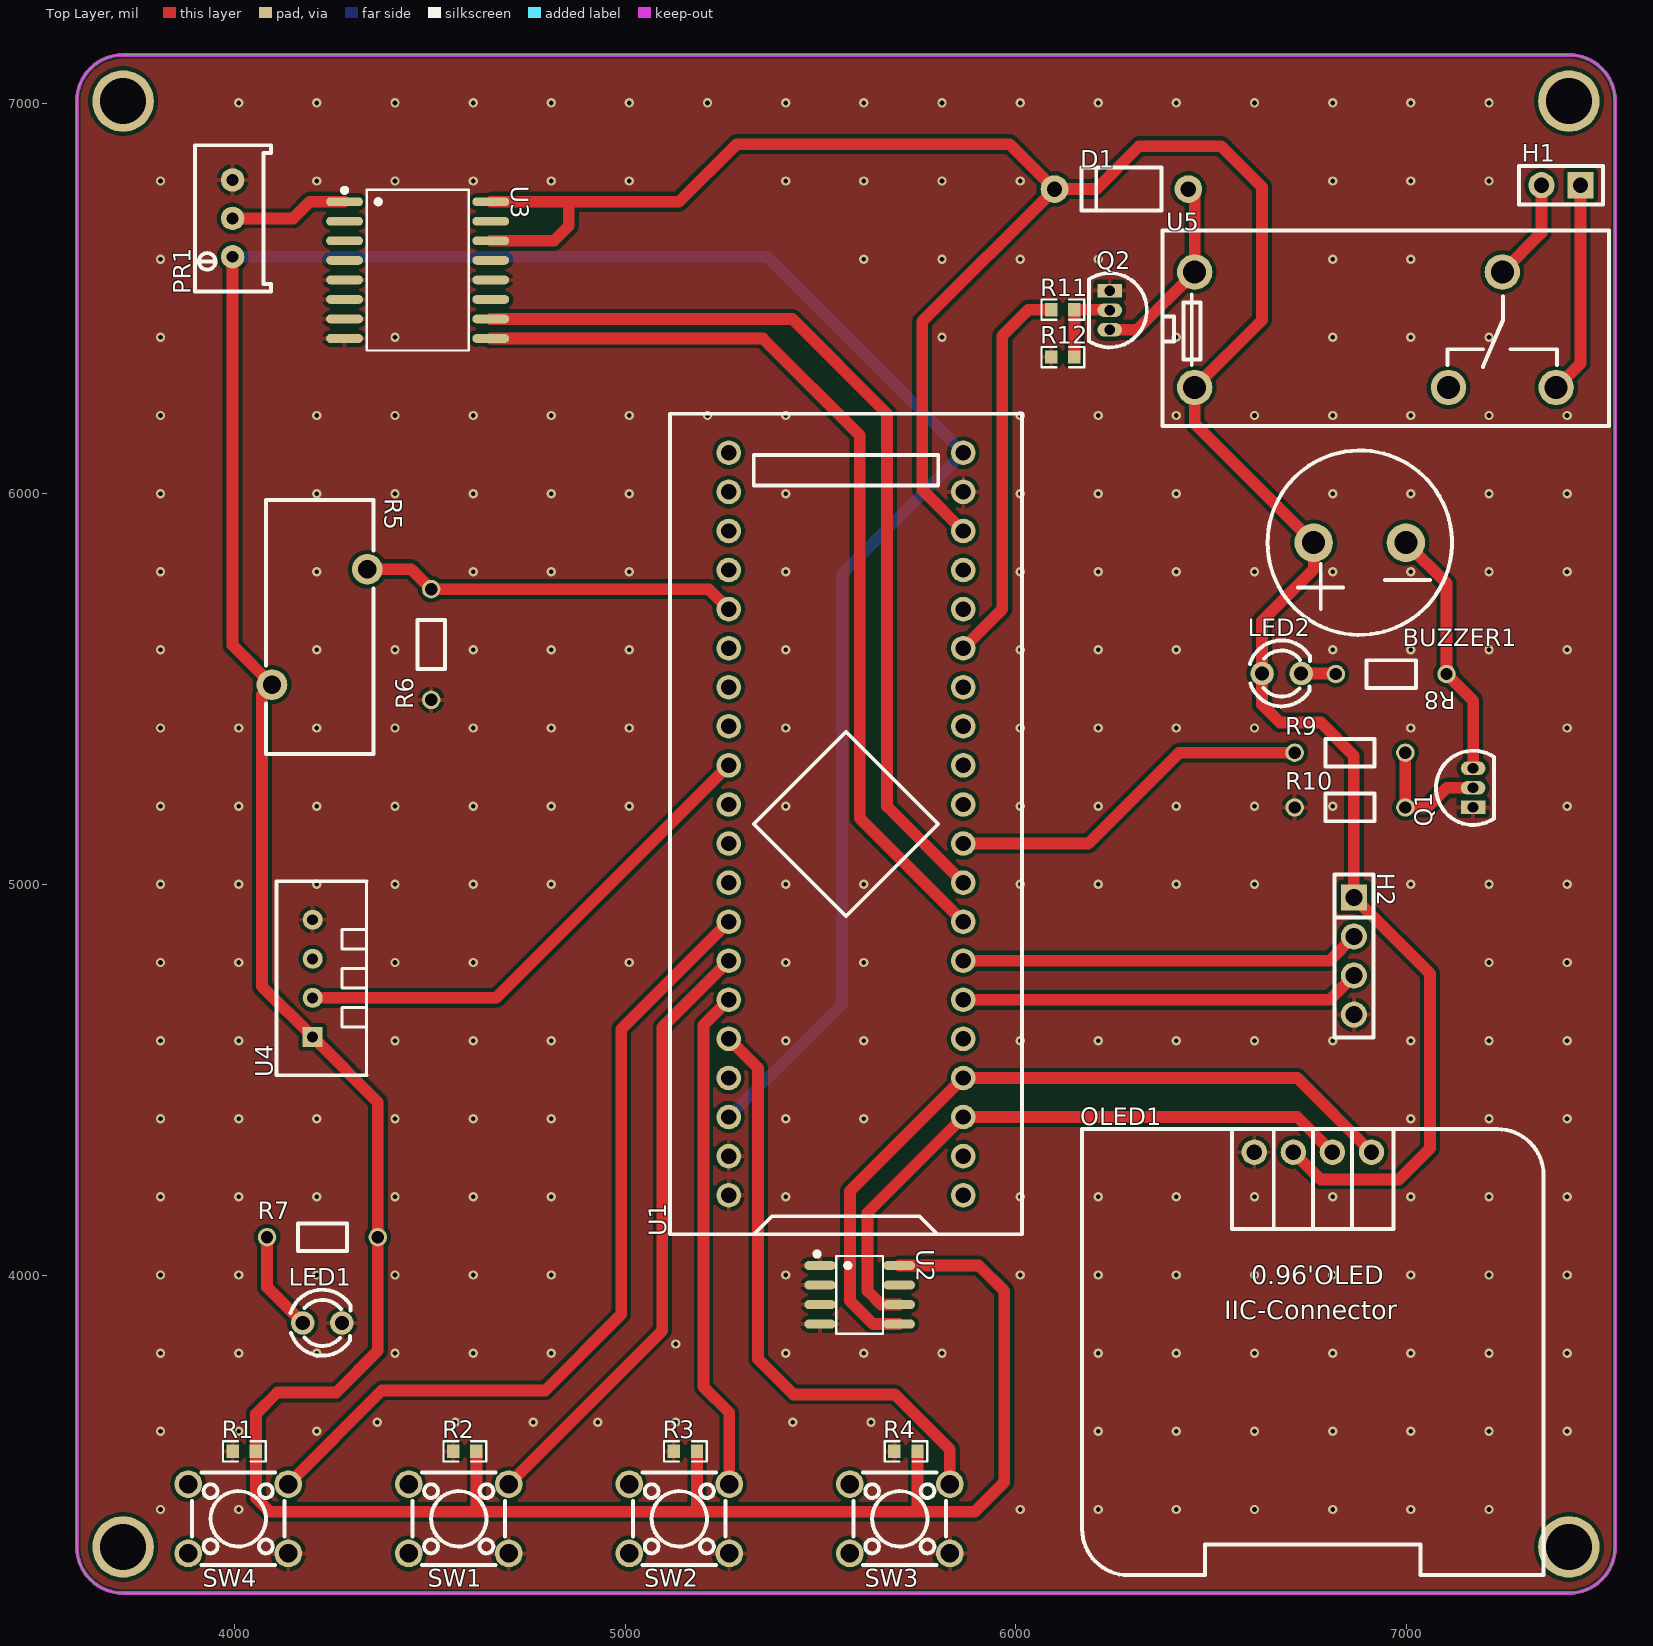
[diagram p0: Top Layer view]
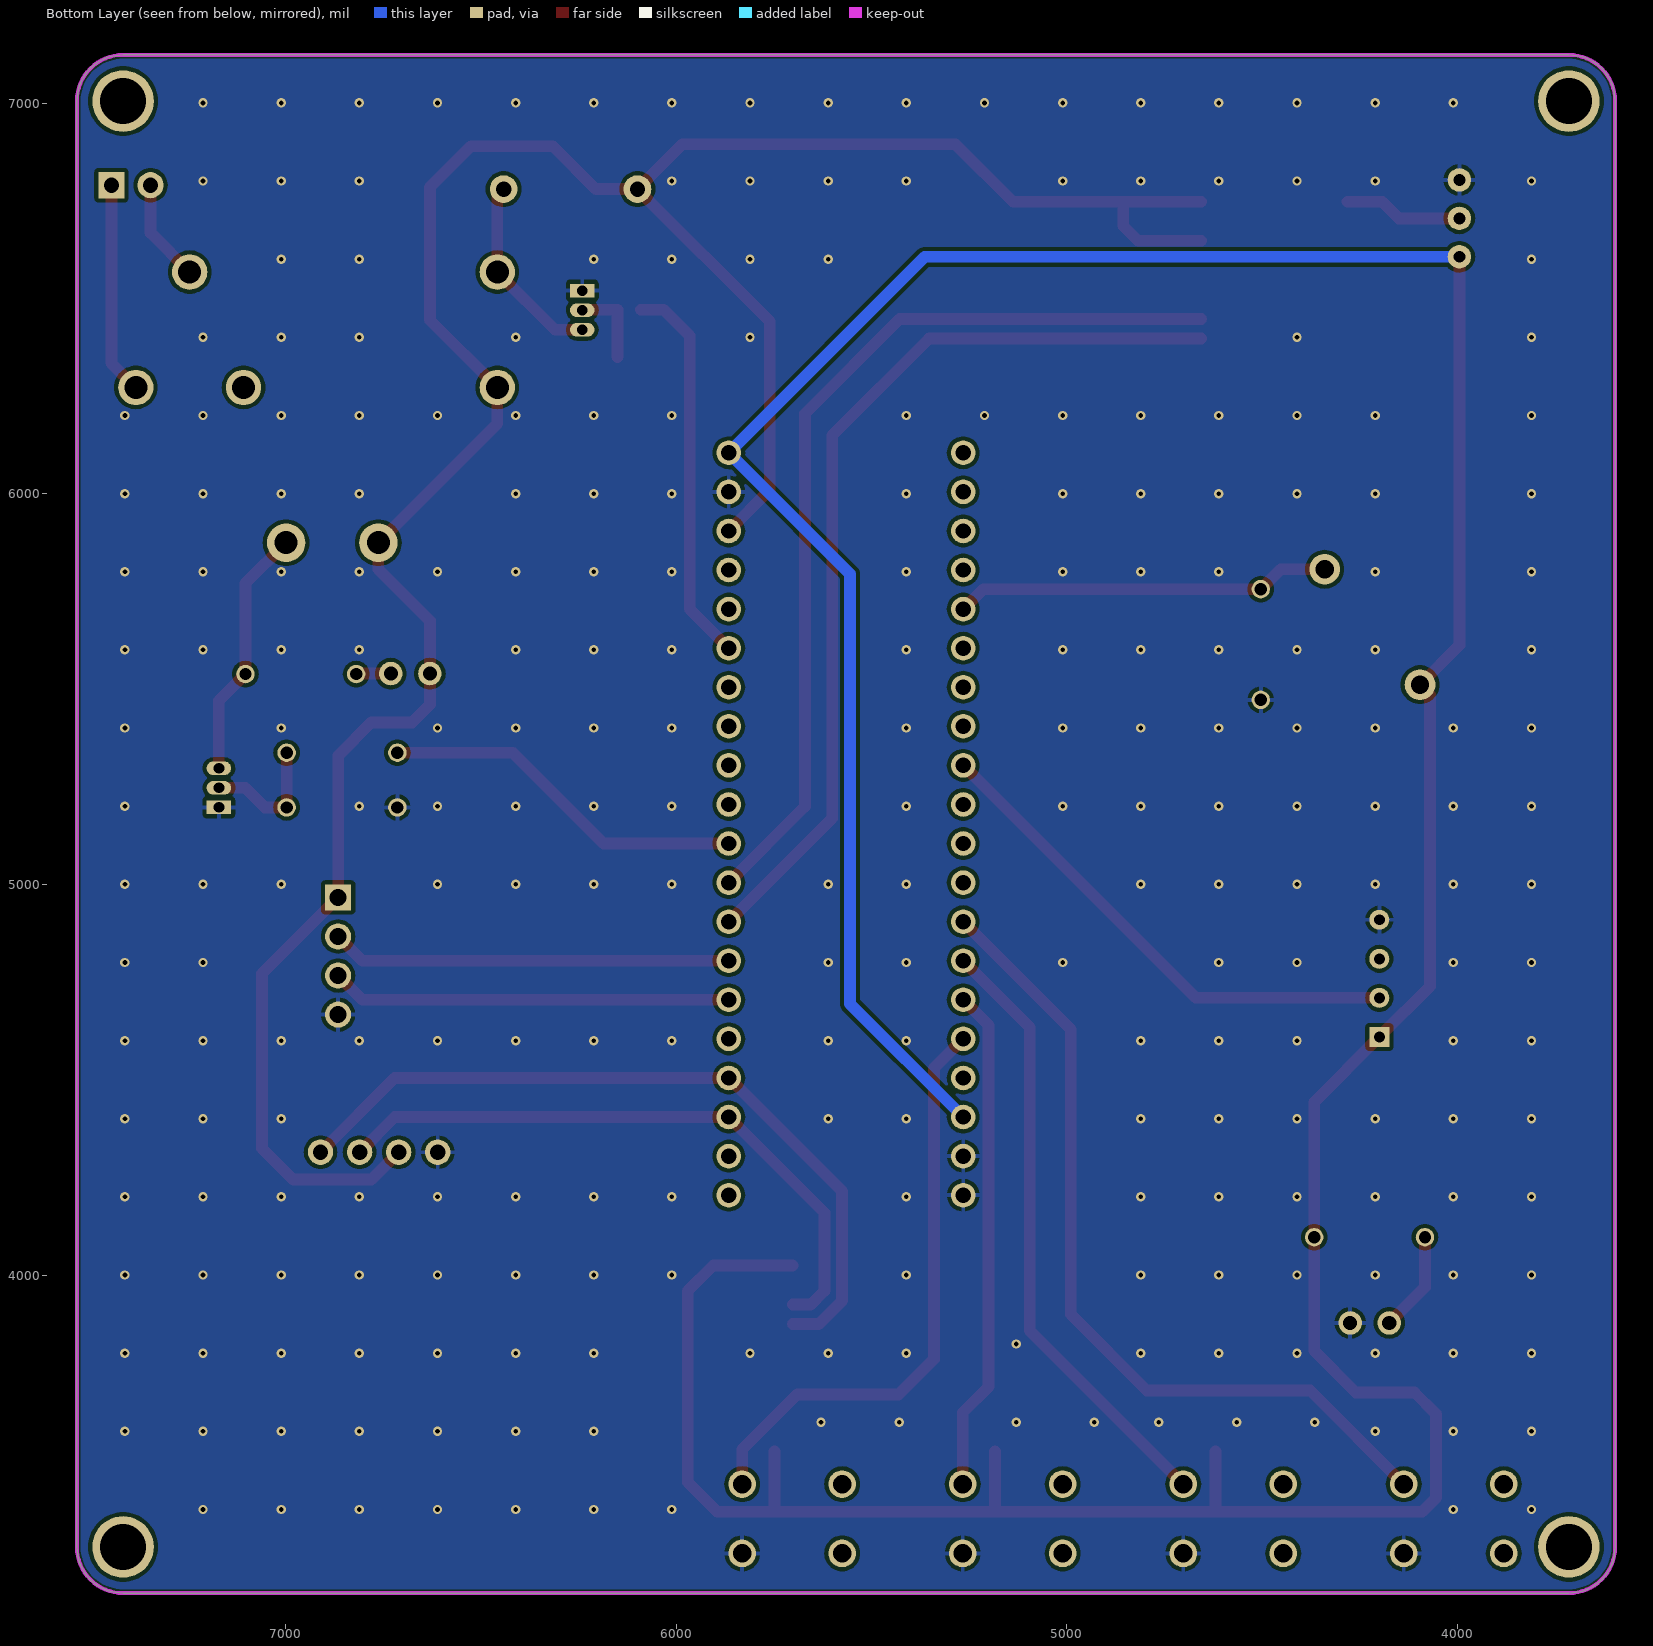
[diagram p1: Bottom Layer view, seen from below]
# Altium PCB MISC75094.pcbdoc
Units mil, origin at the board's own origin, x right, y up, seen from the top; angles counter-clockwise.
Board outline 3937.01 x 3937.01 mil, 2 copper layers (Top Layer, Bottom Layer), stack 62.206 mil thick; 31 components, 46 nets, 144 pads, 253 vias.

## Layer stack, top to bottom
Top Solder Mask Layer: solder mask 0.394, Dk 3.3
Top Layer: signal copper 1.379
Dielectric1: surface 59.449, FR4, Dk 4.5
Bottom Layer: signal copper 1.378
Bottom Solder Mask Layer: solder mask 0.394, Dk 3.3

## Board outline
3714.61,7123.5 ccw(c3714.61,7005.39) 3596.5,7005.39 3596.5,3304.61 ccw(c3714.61,3304.61) 3714.61,3186.5 7415.39,3186.5 ccw(c7415.39,3304.61) 7533.5,3304.61 7533.5,7005.39 ccw(c7415.39,7005.39) 7415.39,7123.5 3714.61,7123.5

## Design rules (kind name [scope] priority, off if disabled: settings)
BoardOutlineClearance copperThickness2oz_1 [All] p2 off: genericclearance=7.99 ignorepadtopadclearanceinfootprint=FALSE except(0: Arc-SplitContinuation Track-SplitContinuation SMDPad-SplitContinuation THPad-SplitContinuation Via-SplitContinuation Fill-SplitContinuation Region-SplitContinuation Poly-SplitContinuation Text-SplitContinuation Hole-SplitContinuation; 5.98: Arc-CutoutEdge Track-CutoutEdge SMDPad-CutoutEdge THPad-CutoutEdge Via-CutoutEdge Text-CutoutEdge; 6.9: Hole-OutlineEdge Hole-CutoutEdge; 10: Poly-OutlineEdge Poly-CutoutEdge; 11.81: Arc-OutlineEdge Track-OutlineEdge SMDPad-OutlineEdge THPad-OutlineEdge Via-OutlineEdge Fill-OutlineEdge Region-OutlineEdge Text-OutlineEdge Fill-CutoutEdge Region-CutoutEdge)
BoardOutlineClearance Plane_innerPlane_1 [All] p4 off: genericclearance=4.02 ignorepadtopadclearanceinfootprint=FALSE except(0: Arc-SplitContinuation Track-SplitContinuation SMDPad-SplitContinuation THPad-SplitContinuation Via-SplitContinuation Fill-SplitContinuation Region-SplitContinuation Poly-SplitContinuation Text-SplitContinuation Hole-SplitContinuation; 5.98: Arc-CutoutEdge Track-CutoutEdge SMDPad-CutoutEdge THPad-CutoutEdge Via-CutoutEdge Text-CutoutEdge; 6.9: Hole-OutlineEdge Hole-CutoutEdge; 10: Poly-OutlineEdge Poly-CutoutEdge; 11.81: Arc-OutlineEdge Track-OutlineEdge SMDPad-OutlineEdge THPad-OutlineEdge Via-OutlineEdge Fill-OutlineEdge Region-OutlineEdge Text-OutlineEdge Fill-CutoutEdge Region-CutoutEdge)
BoardOutlineClearance Copper_copperRegion_1 [All] p6 off: genericclearance=4.02 ignorepadtopadclearanceinfootprint=FALSE except(0: Arc-SplitContinuation Track-SplitContinuation SMDPad-SplitContinuation THPad-SplitContinuation Via-SplitContinuation Fill-SplitContinuation Region-SplitContinuation Poly-SplitContinuation Text-SplitContinuation Hole-SplitContinuation; 5.98: Arc-CutoutEdge Track-CutoutEdge SMDPad-CutoutEdge THPad-CutoutEdge Via-CutoutEdge Text-CutoutEdge; 6.9: Hole-OutlineEdge Hole-CutoutEdge; 10: Poly-OutlineEdge Poly-CutoutEdge; 11.81: Arc-OutlineEdge Track-OutlineEdge SMDPad-OutlineEdge THPad-OutlineEdge Via-OutlineEdge Fill-OutlineEdge Region-OutlineEdge Text-OutlineEdge Fill-CutoutEdge Region-CutoutEdge)
BoardOutlineClearance copperThickness1oz_1 [All] p8: genericclearance=4.02 ignorepadtopadclearanceinfootprint=FALSE except(0: Arc-SplitContinuation Track-SplitContinuation SMDPad-SplitContinuation THPad-SplitContinuation Via-SplitContinuation Fill-SplitContinuation Region-SplitContinuation Poly-SplitContinuation Text-SplitContinuation Hole-SplitContinuation; 5.98: Arc-CutoutEdge Track-CutoutEdge SMDPad-CutoutEdge THPad-CutoutEdge Via-CutoutEdge Text-CutoutEdge; 6.9: Hole-OutlineEdge Hole-CutoutEdge; 10: Poly-OutlineEdge Poly-CutoutEdge; 11.81: Arc-OutlineEdge Track-OutlineEdge SMDPad-OutlineEdge THPad-OutlineEdge Via-OutlineEdge Fill-OutlineEdge Region-OutlineEdge Text-OutlineEdge Fill-CutoutEdge Region-CutoutEdge)
Clearance copperThickness2oz [All] p1 off: gap=7.99 ignorepadtopadclearanceinfootprint=FALSE except(5.98: SMDPad-Track SMDPad-SMDPad THPad-Track SMDPad-THPad THPad-THPad Track-Via SMDPad-Via THPad-Via Via-Via Fill-SMDPad Region-SMDPad Fill-THPad Region-THPad Fill-Via Region-Via Fill-Fill Fill-Region Region-Region Arc-Track Arc-SMDPad Arc-THPad Arc-Via Fill-Arc Region-Arc Arc-Arc Text-Track SMDPad-Text Text-THPad Text-Via Fill-Text Region-Text Arc-Text Text-Text; 6.9: Hole-Track Hole-SMDPad Hole-THPad Hole-Via Fill-Hole Region-Hole Hole-Arc Hole-Text; 10: Poly-Track Poly-SMDPad Poly-THPad Poly-Via Poly-Fill Poly-Region Poly-Poly Poly-Arc Poly-Text Poly-Hole; 11.81: Fill-Track Region-Track)
Clearance Plane_innerPlane [All] p3 off: gap=4.02 ignorepadtopadclearanceinfootprint=FALSE except(5.98: SMDPad-Track SMDPad-SMDPad THPad-Track SMDPad-THPad THPad-THPad Track-Via SMDPad-Via THPad-Via Via-Via Fill-SMDPad Region-SMDPad Fill-THPad Region-THPad Fill-Via Region-Via Fill-Fill Fill-Region Region-Region Arc-Track Arc-SMDPad Arc-THPad Arc-Via Fill-Arc Region-Arc Arc-Arc Text-Track SMDPad-Text Text-THPad Text-Via Fill-Text Region-Text Arc-Text Text-Text; 6.9: Hole-Track Hole-SMDPad Hole-THPad Hole-Via Fill-Hole Region-Hole Hole-Arc Hole-Text; 10: Poly-Track Poly-SMDPad Poly-THPad Poly-Via Poly-Fill Poly-Region Poly-Poly Poly-Arc Poly-Text Poly-Hole; 11.81: Fill-Track Region-Track)
Clearance Copper_copperRegion [All] p5 off: gap=4.02 ignorepadtopadclearanceinfootprint=FALSE except(5.98: SMDPad-Track SMDPad-SMDPad THPad-Track SMDPad-THPad THPad-THPad Track-Via SMDPad-Via THPad-Via Via-Via Fill-SMDPad Region-SMDPad Fill-THPad Region-THPad Fill-Via Region-Via Fill-Fill Fill-Region Region-Region Arc-Track Arc-SMDPad Arc-THPad Arc-Via Fill-Arc Region-Arc Arc-Arc Text-Track SMDPad-Text Text-THPad Text-Via Fill-Text Region-Text Arc-Text Text-Text; 6.9: Hole-Track Hole-SMDPad Hole-THPad Hole-Via Fill-Hole Region-Hole Hole-Arc Hole-Text; 10: Poly-Track Poly-SMDPad Poly-THPad Poly-Via Poly-Fill Poly-Region Poly-Poly Poly-Arc Poly-Text Poly-Hole; 11.81: Fill-Track Region-Track)
Clearance copperThickness1oz [All] p7: gap=4.02 ignorepadtopadclearanceinfootprint=FALSE except(5.98: SMDPad-Track SMDPad-SMDPad THPad-Track SMDPad-THPad THPad-THPad Track-Via SMDPad-Via THPad-Via Via-Via Fill-SMDPad Region-SMDPad Fill-THPad Region-THPad Fill-Via Region-Via Fill-Fill Fill-Region Region-Region Arc-Track Arc-SMDPad Arc-THPad Arc-Via Fill-Arc Region-Arc Arc-Arc Text-Track SMDPad-Text Text-THPad Text-Via Fill-Text Region-Text Arc-Text Text-Text; 6.9: Hole-Track Hole-SMDPad Hole-THPad Hole-Via Fill-Hole Region-Hole Hole-Arc Hole-Text; 10: Poly-Track Poly-SMDPad Poly-THPad Poly-Via Poly-Fill Poly-Region Poly-Poly Poly-Arc Poly-Text Poly-Hole; 11.81: Fill-Track Region-Track)
DiffPairsRouting differentialPair [All] p1: maxlimit=6 minlimit=6 mostfreqgap=6 toplayer_minwidth=5 toplayer_prefwidth=10 toplayer_maxwidth=100 toplayer_mingap=6 toplayer_prefgap=6 toplayer_maxgap=6 bottomlayer_minwidth=5 bottomlayer_prefwidth=10 bottomlayer_maxwidth=100 bottomlayer_mingap=6 bottomlayer_prefgap=6 bottomlayer_maxgap=6 maxuncoupledlength=10
HoleToHoleClearance otherClearance [All] p1: gap=11.81 allowstackedmicrovias=TRUE
Length netLength [All] p1: minlimit=0 maxlimit=0
PasteMaskExpansion pasteMaskExpansion [All] p1: expansion=0
PlaneConnect innerPlane [All] p1: planeconnectstyle=Relief reliefexpansion=20 reliefentries=4 reliefconductorwidth=10 reliefairgap=10
PolygonConnect copperRegion [All] p1: connectstyle=Relief reliefconductorwidth=10 reliefentries=4 polygonreliefangle="90 Angle" airgapwidth=10 via.connectstyle=Relief via.reliefconductorwidth=10 via.reliefentries=4 via.polygonreliefangle="90 Angle" via.airgapwidth=10
RoutingVias viaSize [All] p1: holewidth=12.01 width=24.02 viastyle="Through Hole" minholewidth=11.81 minwidth=19.68 maxholewidth=248.03 maxwidth=393.7
SolderMaskExpansion solderMaskExpansion [IsVia] p1: expansion=-1000 istentingtop=TRUE
SolderMaskExpansion solderMaskExpansion [All] p2: expansion=2 istentingtop=FALSE
Width copperThickness2oz_2 [All] p1 off: maxlimit=100 minlimit=8 preferedwidth=10
Width copperThickness1oz_2 [All] p2: maxlimit=100 minlimit=5 preferedwidth=10

## Components (designator, comment, footprint, x,y, rotation, side; value= is the part's Value field where it differs from the comment)
BUZZER1 "buzzer" BUZ-TH_BD12.0-P6.00-D0.9-RD 6880,5875 r180 top
D1 "" DO_1N4007 6270,6780 r0 top
H1 "" HDR-TH_2P-P2.54-V-F 7395,6790 r180 top
H2 "" HDR-TH_4P-P2.54-V-F 6864.9,4817.04 r270 top
LED1 "" LED_TH-3mm 4224.65,3877.95 r0 top
LED2 "" LED_TH-3mm 6680,5540 r0 top
OLED1 "" 0.96OLED_4P 6760,4315 r0 top
PR1 "10kΩ" R_3296 3990,6705 r90 top
Q1 "" S8050_TO_92 7170.1,5247.66 r90 top
Q2 "" S8050_TO_92 6240,6470 r270 top
R1 "10K" R0603 4025.08,3549.45 r0 top
R2 "10K" R0603 4589.49,3549.45 r0 top
R3 "10K" R0603 5153.9,3549.45 r0 top
R4 "10K" R0603 5718.32,3549.45 r0 top
R5 "3Ω,7A,0.075Ω" RES-TH_L16.5-W7.0-P7.50-D0.8-S6.2 4217.88,5659.29 r270 top
R6 "10kΩ" Res_1/8W 4505.81,5614.38 r90 top
R7 "500Ω" Res_1/8W 4225,4095 r0 top
R8 "10Ω" Res_1/8W 6960.41,5541.25 r180 top
R9 "1kΩ" Res_1/8W 6855,5335 r0 top
R10 "10kΩ" Res_1/8W 6855,5195 r0 top
R11 "1K" R0603 6119.85,6471.25 r0 top
R12 "10K" R0603 6120,6350 r0 top
SW1 "" SW-TH_4P-L6.0-W6.0-P4.50-LS6.5 4573.89,3376.74 r180 top
SW2 "" SW-TH_4P-L6.0-W6.0-P4.50-LS6.5 5138.3,3376.74 r180 top
SW3 "" SW-TH_4P-L6.0-W6.0-P4.50-LS6.5 5702.72,3376.74 r180 top
SW4 "" SW-TH_4P-L6.0-W6.0-P4.50-LS6.5 4009.48,3376.74 r180 top
U1 "STM32F103C8T6-Card" CONN-TH_L53.3-W22.9_STM32F103C8T6-CARD 5565,5155 r90 top
U2 "24C02CT-I/SN" SOIC-8_L4.9-W3.9-P1.27-LS6.0-BL 5600,3950 r270 top
U3 "PCF8591T" SOIC-16_L10.3-W7.5-P1.27-LS10.3-BL 4468.71,6572.61 r270 top
U4 "DHT11" SENSOR-TH_DHT11 4200,4760 r90 top
U5 "SSKD6132" RELAY-TH_G2R-1 6920,6420 r0 top

## Footprints (in the part's own frame and the unit in brackets; to place one, negate y for a bottom-side part, rotate by r counter-clockwise, add the part's x,y. Pads: shape width x height; smd on the part's side, far side on the other; paste and mask are expansions set on the pad)
0.96OLED_4P [mm]
  round 1.65 hole 1 copper offset 0,0: 1(-3.81,-0.001) 2(-1.27,0.002) 3(1.27,0.002) 4(3.81,0.002)
  silkscreen extent -15,-27.5 15,1.5
BUZ-TH_BD12.0-P6.00-D0.9-RD [mm]
  round 2.5 hole 1.5 paste+0 mask+0.05: 1(-3,0) 2(3,0)
  silkscreen extent -5.99,-5.99 5.99,5.99
CONN-TH_L53.3-W22.9_STM32F103C8T6-CARD [mm]
  round 1.6 hole 1: 1(-24.13,-7.62) 2(-21.59,-7.62) 3(-19.05,-7.62) 4(-16.51,-7.62) 5(-13.97,-7.62) 6(-11.43,-7.62) 7(-8.89,-7.62) 8(-6.35,-7.62) 9(-3.81,-7.62) 10(-1.27,-7.62) 11(1.27,-7.62) 12(3.81,-7.62) 13(6.35,-7.62) 14(8.89,-7.62) 15(11.43,-7.62) 16(13.97,-7.62) 17(16.51,-7.62) 18(19.05,-7.62) 19(21.59,-7.62) 20(24.13,-7.62) 21(24.13,7.62) 22(21.59,7.62) 23(19.05,7.62) 24(16.51,7.62) 25(13.97,7.62) 26(11.43,7.62) 27(8.89,7.62) 28(6.35,7.62) 29(3.81,7.62) 30(1.27,7.62) 31(-1.27,7.62) 32(-3.81,7.62) 33(-6.35,7.62) 34(-8.89,7.62) 35(-11.43,7.62) 36(-13.97,7.62) 37(-16.51,7.62) 38(-19.05,7.62) 39(-21.59,7.62) 40(-24.13,7.62)
  silkscreen extent -26.67,-11.43 26.67,11.43
DO_1N4007 [mm]
  round 1.8 hole 1 paste+0 mask+0.051: 1(-4.35,0) 2(4.35,0)
  silkscreen extent -2.6,-1.4 2.6,1.4
HDR-TH_2P-P2.54-V-F [mm]
  rect 1.7x1.7 hole 1: 1(-1.27,0)
  round 1.7 hole 1: 2(1.27,0)
  silkscreen extent -2.74,-1.25 2.74,1.25
HDR-TH_4P-P2.54-V-F [mm]
  rect 1.7x1.7 hole 1.1: 1(-3.81,0)
  round 1.7 hole 1.1: 2(-1.27,0) 3(1.27,0) 4(3.81,0)
  silkscreen extent -5.29,-1.27 5.29,1.27
LED_TH-3mm [mil]
  round 60 hole 36 paste+0 mask+2: 1(-50,0) 2(50,0)
  silkscreen extent -81,-84 72,85
R0603 [mil]
  rect 31.75x34.02 smd paste-3937.01 mask+2: 1(-29.66,0) 2(29.66,0)
  silkscreen extent -55,-26 55,26
R_3296 [mil]
  round 60 hole 30 paste+0 mask+2: 1(-98.4,-5) 2(0,-5) 3(98.4,-5)
  silkscreen extent -187,-103 187,92
RELAY-TH_G2R-1 [mm]
  round 2.3 hole 1.5: 1(-11.75,-3.75) 2(4.75,-3.75) 3(11.75,-3.75) 4(8.25,3.75) 5(-11.75,3.75)
  silkscreen extent -13.83,-6.26 15.17,6.44
RES-TH_L16.5-W7.0-P7.50-D0.8-S6.2 [mm]
  round 2 hole 1.2: 1(-3.75,3.1) 2(3.75,-3.1)
  silkscreen extent -8.25,-3.5 8.25,3.5
Res_1/8W [mil]
  round 47.2 hole 31.5 paste+0 mask+2: 1(-141.7,2.48) 2(141.7,2.48)
  silkscreen extent -63,-33 63,38
S8050_TO_92 [mil]
  rect 35.4x63 hole 27.6 paste+0 mask+2: 1(-50,0)
  oval 35.4x63 hole 27.6 paste+0 mask+2: 2(0,0) 3(50,0)
  silkscreen extent -95,-53 95,95
SENSOR-TH_DHT11 [mil]
  rect 51x51 hole 28: 1(-150,0)
  round 51 hole 28: 2(-50,0) 3(50,0) 4(150,0)
  silkscreen extent -248,-138 248,93
SOIC-8_L4.9-W3.9-P1.27-LS6.0-BL [mm]
  oval 0.588x2.045 smd: 1(-1.905,-2.57) 2(-0.635,-2.57) 3(0.635,-2.57) 4(1.905,-2.57) 5(1.905,2.57) 6(0.635,2.57) 7(-0.635,2.57) 8(-1.905,2.57)
  silkscreen extent -2.8,-2.92 2.53,1.52
SOIC-16_L10.3-W7.5-P1.27-LS10.3-BL [mil]
  oval 22.6x94.51 smd: 1(-175,-187.02) 2(-125,-187.02) 3(-75,-187.02) 4(-25,-187.02) 5(25,-187.02) 6(75,-187.02) 7(125,-187.02) 8(175,-187.02) 9(175,187.02) 10(125,187.02) 11(75,187.02) 12(25,187.02) 13(-25,187.02) 14(-75,187.02) 15(-125,187.02) 16(-175,187.02)
  silkscreen extent -210,-193 206,131
SW-TH_4P-L6.0-W6.0-P4.50-LS6.5 [mm]
  round 1.8 hole 1.2: 1(-3.25,2.25) 2(3.25,2.25) 3(-3.25,-2.25) 4(3.25,-2.25)
  silkscreen extent -3,-3 3,3

## Free pads (board coordinates)
  round 157.48 hole 118.11: 1(3714.61,7005.39) 1(3714.61,3304.61) 1(7415.39,7005.39) 1(7415.39,3304.61)

## Via types
v1: diameter 24.02, hole 12, Top Layer to Bottom Layer, 253 vias

## Nets (pads, with @x,y where several pads share a name; then routed paths per layer and width w, separated by ;. In a path a pad name is that pad's centre, name@x,y a point inside that pad or via, vN(x,y) a via of type N, cw(c..) or ccw(c..) an arc to the next point about the centre after c; other vN are vias at no path point)
$1N17153: LED1.1 R7.1 | length 257.4
  Top Layer w30: R7.1 4083.3,3969.3 LED1.1
$1N17160: PR1.2 U3.1 | length 314.3
  Top Layer w30: PR1.2@3985,6705 4150,6705 4192.61,6747.61 U3.1
$1N17168: BUZZER1.1 Q1.3 R8.1 | length 648.6
  Top Layer w30: BUZZER1.1 7102.11,5771 R8.1 7170.1,5470.79 Q1.3
$1N17169: Q1.2 R9.2 R10.2 | length 334.2
  Top Layer w30: R9.2 R10.2 7052.48,5197.48 7102.66,5247.66 Q1.2
$1N17173: LED2.2 R8.2 | length 89.2
  Top Layer w30: LED2.2 6817.49,5540 R8.2
$1N17174: D1.2 Q2.3 U5.5 | length 497.6
  Top Layer w30: Q2.3 6309.75,6420 U5.5 6457.4,6763.86 D1.2
$1N17176: Q2.2 R11.2 R12.2 | length 212.3
  Top Layer w30: R12.2 6149.66,6471.1 R11.2 6238.75,6471.25 Q2.2
$1N17179: H1.2 U5.4 | length 263.9
  Top Layer w30: U5.4 7345,6667.85 H1.2
$1N17180: H1.1 U5.3 | length 543.5
  Top Layer w30: U5.3 7445,6334.75 H1.1
+5V: BUZZER1.2 D1.1 H2.1 LED2.1 OLED1.2 U1.18 U3.14 U3.16 U5.1 | length 6872.4
  Top Layer w30: U3.14 4817.61,6647.61 4855.55,6685.55 4855.55,6747.61 ; U3.16 4855.55,6747.61 ; U1.18 5760,6010 5760,6441.26 D1.1 ; OLED1.2@6710,4315.05 6780.05,4245 6980,4245 7060,4325 7060,4771.94 H2.1 6864.9,5330.1 6780,5415 6675,5415 6630,5460 LED2.1 6630,5675 6761.89,5806.89 BUZZER1.2 6457.4,6179.49 U5.1 6630,6444.95 6630,6785 6525,6890 6315,6890 6205,6780 D1.1 ; 4855.55,6747.61 5137.61,6747.61 5285,6895 5983.74,6895 D1.1
BUZZER: R9.1 U1.10 | length 944.6
  Top Layer w30: U1.10 6185,5105 6417.48,5337.48 R9.1
DATA: U1.29 U4.2 | length 1311.5
  Top Layer w30: U4.2 4670,4710 U1.29
GND: H2.4 LED1.2 OLED1.1 PR1.3 Q1.1 Q2.1 R1.1 R2.1 R3.1 R4.1 R6.1 R10.1 R12.1 SW1.1 SW2.1 SW3.1 SW4.1 U1.19 U1.39 U1.40 U2.1 U2.2 U2.3 U2.4 U3.5 U3.6 U3.7 U3.8 U3.12 U4.4
  other v1: 3810.6,3400.6 4010.6,3400.6 6010.6,3400.6 6210.6,3400.6 6410.6,3400.6 6610.6,3400.6 6810.6,3400.6 7010.6,3400.6 7210.6,3400.6 3810.6,3600.6 4010.6,3600.6 4210.6,3600.6 6210.6,3600.6 6410.6,3600.6 6610.6,3600.6 6810.6,3600.6 7010.6,3600.6 7210.6,3600.6 7410.6,3600.6 4364.89,3624.1 4564.89,3624.1 4764.89,3624.1 4929.3,3624.1 5129.3,3624.1 5429.1,3624.1 5629.1,3624.1 3810.6,3800.6 4010.6,3800.6 4210.6,3800.6 4410.6,3800.6 4610.6,3800.6 4810.6,3800.6 5410.6,3800.6 5610.6,3800.6 5810.6,3800.6 6210.6,3800.6 6410.6,3800.6 6610.6,3800.6 6810.6,3800.6 7010.6,3800.6 7210.6,3800.6 7410.6,3800.6 5129.3,3824.1 3810.6,4000.6 4010.6,4000.6 4210.6,4000.6 4410.6,4000.6 4610.6,4000.6 4810.6,4000.6 5410.6,4000.6 6010.6,4000.6 6210.6,4000.6 6410.6,4000.6 6610.6,4000.6 6810.6,4000.6 7010.6,4000.6 7210.6,4000.6 7410.6,4000.6 3810.6,4200.6 4010.6,4200.6 4210.6,4200.6 4410.6,4200.6 4610.6,4200.6 4810.6,4200.6 5410.6,4200.6 6010.6,4200.6 6210.6,4200.6 6410.6,4200.6 6610.6,4200.6 6810.6,4200.6 7010.6,4200.6 7210.6,4200.6 7410.6,4200.6 3810.6,4400.6 4010.6,4400.6 4210.6,4400.6 4410.6,4400.6 4610.6,4400.6 4810.6,4400.6 5410.6,4400.6 5610.6,4400.6 7010.6,4400.6 7210.6,4400.6 7410.6,4400.6 3810.6,4600.6 4010.6,4600.6 4410.6,4600.6 4610.6,4600.6 4810.6,4600.6 5410.6,4600.6 5610.6,4600.6 6010.6,4600.6 6210.6,4600.6 6410.6,4600.6 6610.6,4600.6 6810.6,4600.6 7010.6,4600.6 7210.6,4600.6 7410.6,4600.6 3810.6,4800.6 4010.6,4800.6 4410.6,4800.6 4610.6,4800.6 5010.6,4800.6 5410.6,4800.6 5610.6,4800.6 7210.6,4800.6 7410.6,4800.6 3810.6,5000.6 4010.6,5000.6 4210.6,5000.6 4410.6,5000.6 4610.6,5000.6 4810.6,5000.6 5410.6,5000.6 5610.6,5000.6 6010.6,5000.6 6210.6,5000.6 6410.6,5000.6 6610.6,5000.6 7010.6,5000.6 7210.6,5000.6 7410.6,5000.6 3810.6,5200.6 4010.6,5200.6 4210.6,5200.6 4410.6,5200.6 4610.6,5200.6 4810.6,5200.6 5010.6,5200.6 5410.6,5200.6 6010.6,5200.6 6210.6,5200.6 6410.6,5200.6 6610.6,5200.6 6810.6,5200.6 7410.6,5200.6 3810.6,5400.6 4010.6,5400.6 4210.6,5400.6 4410.6,5400.6 4610.6,5400.6 4810.6,5400.6 5010.6,5400.6 5410.6,5400.6 6010.6,5400.6 6210.6,5400.6 6410.6,5400.6 6610.6,5400.6 7010.6,5400.6 7410.6,5400.6 3810.6,5600.6 4210.6,5600.6 4410.6,5600.6 4610.6,5600.6 4810.6,5600.6 5010.6,5600.6 5410.6,5600.6 6010.6,5600.6 6210.6,5600.6 6410.6,5600.6 6810.6,5600.6 7010.6,5600.6 7210.6,5600.6 7410.6,5600.6 3810.6,5800.6 4210.6,5800.6 4610.6,5800.6 4810.6,5800.6 5010.6,5800.6 5410.6,5800.6 6010.6,5800.6 6210.6,5800.6 6410.6,5800.6 6610.6,5800.6 6810.6,5800.6 7010.6,5800.6 7210.6,5800.6 7410.6,5800.6 3810.6,6000.6 4210.6,6000.6 4410.6,6000.6 4610.6,6000.6 4810.6,6000.6 5010.6,6000.6 5410.6,6000.6 6010.6,6000.6 6210.6,6000.6 6410.6,6000.6 6810.6,6000.6 7010.6,6000.6 7210.6,6000.6 7410.6,6000.6 3810.6,6200.6 4210.6,6200.6 4410.6,6200.6 4610.6,6200.6 4810.6,6200.6 5010.6,6200.6 5210.6,6200.6 5410.6,6200.6 6010.6,6200.6 6210.6,6200.6 6410.6,6200.6 6610.6,6200.6 6810.6,6200.6 7010.6,6200.6 7210.6,6200.6 7410.6,6200.6 3810.6,6400.6 4410.6,6400.6 5810.6,6400.6 6410.6,6400.6 6810.6,6400.6 7010.6,6400.6 7210.6,6400.6 3810.6,6600.6 5610.6,6600.6 5810.6,6600.6 6010.6,6600.6 6210.6,6600.6 6810.6,6600.6 7010.6,6600.6 3810.6,6800.6 4210.6,6800.6 4410.6,6800.6 4610.6,6800.6 4810.6,6800.6 5010.6,6800.6 5410.6,6800.6 5610.6,6800.6 5810.6,6800.6 6010.6,6800.6 6810.6,6800.6 7010.6,6800.6 7210.6,6800.6 4010.6,7000.6 4210.6,7000.6 4410.6,7000.6 4610.6,7000.6 4810.6,7000.6 5010.6,7000.6 5210.6,7000.6 5410.6,7000.6 5610.6,7000.6 5810.6,7000.6 6010.6,7000.6 6210.6,7000.6 6410.6,7000.6 6610.6,7000.6 6810.6,7000.6 7010.6,7000.6 7210.6,7000.6
KEY1: SW4.3 U1.33 | length 2151.5
  Top Layer w30: SW4.3 4377.11,3705 4795,3705 4990,3900 4990,4630 U1.33
KEY2: SW1.3 U1.34 | length 1572.9
  Top Layer w30: SW1.3 5095,3858.48 5095,4635 U1.34
KEY3: SW2.3 U1.35 | length 1294
  Top Layer w30: U1.35 5200,4640 5200,3715 5266.25,3648.75 SW2.3
KEY4: SW3.3 U1.36 | length 1526.3
  Top Layer w30: U1.36 5340,4530 5340,3785 5430,3695 5690,3695 5830.67,3554.33 SW3.3
NRST: U1.37
PA0: R5.1 R6.2 U1.25 | length 967.3
  Top Layer w30: R5.1 4452.49,5806.93 R6.2 5213.92,5756.08 U1.25
PA1: U1.26
PA2: U1.27
PA3: U1.28
PA5: U1.30
PA6: U1.31
PA7: U1.32
PA8: U1.5
PB3: U1.11
PB4: U1.12
PB5: U1.13
PB6: U1.14
PB8: U1.16
PB9: U1.17
PB12: U1.1
PB13: U1.2
PC13: U1.22
PC14: U1.23
PC15: U1.24
RELAY: R11.1 U1.15 | length 994
  Top Layer w30: U1.15 5965,5705 5965,6405 6031.25,6471.25 R11.1
RX1: H2.2 U1.7 | length 1025.6
  Top Layer w30: U1.7 6802.86,4805 H2.2
SCL: OLED1.3 U1.3 U2.6 | length 1624.4
  Top Layer w30: U2.6 5655,3925 5620,3960 5620,4160 U1.3 6720.05,4405 OLED1.3@6810,4315.05
SCL1: U1.9 U3.10 | length 2395.5
  Top Layer w30: U3.10 5427.39,6447.61 5670,6205 5670,5200 U1.9
SDA: OLED1.4 U1.4 U2.5 | length 1964.8
  Top Layer w30: U2.5 5635,3875 5575,3935 5575,4215 U1.4 6720.05,4505 OLED1.4@6910,4315.05
SDA1: U1.8 U3.9 | length 2401.6
  Top Layer w30: U3.9 5352.39,6397.61 5600,6150 5600,5170 U1.8
TX1: H2.3 U1.6 | length 1025.6
  Top Layer w30: U1.6 6802.86,4705 H2.3
VBAT: U1.21
VCC: PR1.1 R1.2 R2.2 R3.2 R4.2 R5.2 R7.2 U1.20 U1.38 U2.8 U4.1 | length 10805.9
  Top Layer w30: PR1.1 3995,5612.48 R5.2 4070,5485.82 4070,4740 U4.1 4366.7,4443.3 R7.2 4366.7,3806.7 4260,3700 4110,3700 4054.74,3644.74 R1.2 4054.74,3430.26 4090,3395 4617.77,3395 ; R2.2 4619.15,3396.38 4617.77,3395 ; R3.2 5183.56,3395.52 5183.05,3395 ; U2.8 5905,4025 5970,3960 5970,3470 5895,3395 5747.98,3395 ; R4.2 5747.98,3395 ; 4617.77,3395 5183.05,3395 ; 5183.05,3395 5747.98,3395
  Bottom Layer w30: PR1.1 5363.4,6606.6 U1.20 5555,5795 5555,4695 U1.38
pads on no net: SW1.2 SW1.4 SW2.2 SW2.4 SW3.2 SW3.4 SW4.2 SW4.4 U2.7 U3.2 U3.3 U3.4 U3.11 U3.13 U3.15 U4.3 U5.2

## Polygon pours and split planes (outlines as drawn)
GND on Bottom Layer (solid, remove dead copper, pour order 2): 3525,7245 3525,3080 7700,3080 7700,7245
GND on Top Layer (solid, remove dead copper, pour order 2): 3000,7415 3000,3000 7930,3000 7930,7415

## Keep-outs
Board Outline Layer:
  the board outline again, w10